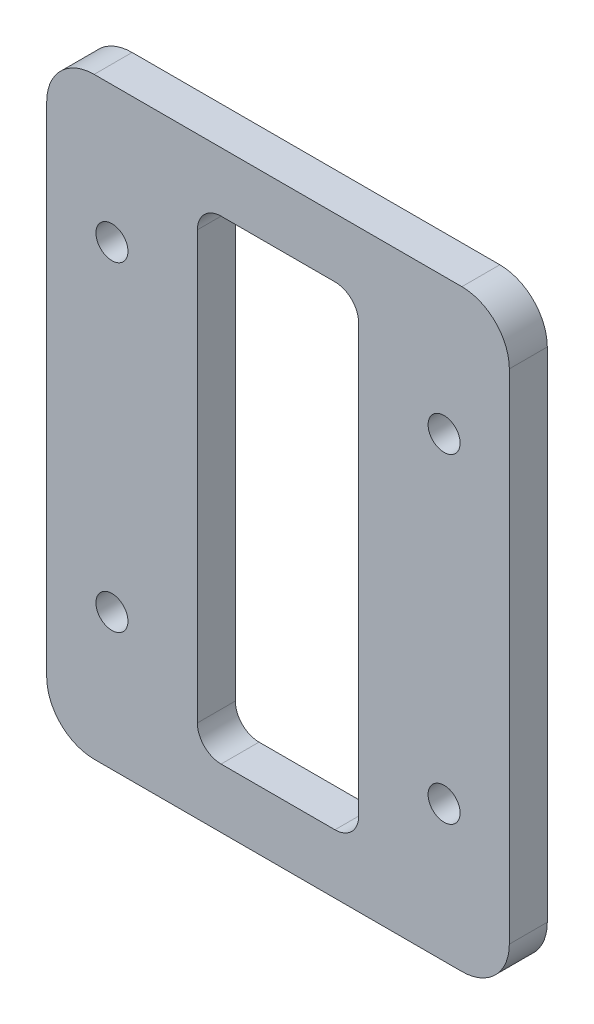
from build123d import *

# Parameters (mm, degrees)
SKETCH1_W           = 195
SKETCH1_H           = 250
SKETCH1_W_2         = 68
SKETCH1_H_2         = 200
BOSS_EXTRUDE1_DEPTH = 8
F_13_5_HOLE1_D      = 13.5
FILLET2_R           = 20
FILLET3_R           = 10


with BuildPart() as part:
    # Sketch1 → Boss-Extrude1 (new, symmetric)
    with BuildSketch(Plane.XY):
        Rectangle(SKETCH1_W, SKETCH1_H)
        Rectangle(SKETCH1_W_2, SKETCH1_H_2, mode=Mode.SUBTRACT)
    extrude(amount=BOSS_EXTRUDE1_DEPTH, both=True)

    # Ø13.5 Hole1 (through all)
    with Locations(Plane.XY.offset(8)):
        with Locations((-70, 67.5), (70, 67.5), (70, -67.5), (-70, -67.5)):
            Hole(F_13_5_HOLE1_D / 2)

    # Fillet2
    fillet2_edges = [part.edges().sort_by_distance(p)[0] for p in [
        (-97.5, 125, 0),
        (97.5, 125, 0),
        (97.5, -125, 0),
        (-97.5, -125, 0),
    ]]
    fillet(fillet2_edges, radius=FILLET2_R)

    # Fillet3
    fillet3_edges = [part.edges().sort_by_distance(p)[0] for p in [
        (-34, 100, 0),
        (-34, -100, 0),
        (34, -100, 0),
        (34, 100, 0),
    ]]
    fillet(fillet3_edges, radius=FILLET3_R)


solid = part.part
